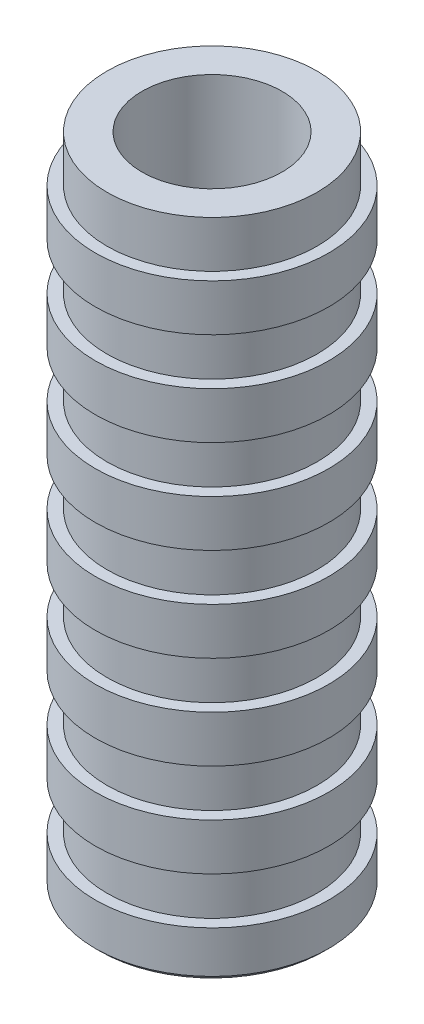
from build123d import *


with BuildPart() as part:
    # 草图1 → 旋转1 (revolve)
    with BuildSketch(Plane(origin=(0, 0, 0), x_dir=(-1, 0, 0), z_dir=(0, 0, -1)), mode=Mode.PRIVATE) as revolve_1_sk:
        Polygon((-22.5, -220), (-25, -220), (-25, -230), (-22.5, -230), (-22.5, -240), (-25, -240), (-25, -250), (-22.5, -250), (-22.5, -260), (-25, -260), (-25, -270), (-22.5, -270), (-22.5, -280), (-25, -280), (-25, -289), (-24, -290), (-16, -290), (-15, -289), (-15, -150), (-22.5, -150), (-22.5, -160), (-25, -160), (-25, -170), (-22.5, -170), (-22.5, -180), (-25, -180), (-25, -190), (-22.5, -190), (-22.5, -200), (-25, -200), (-25, -210), (-22.5, -210), align=None)
    revolve(revolve_1_sk.sketch.rotate(Axis((0, -290, 0), (0, 1, 0)), 270), axis=Axis((0, -290, 0), (0, 1, 0)))


solid = part.part
